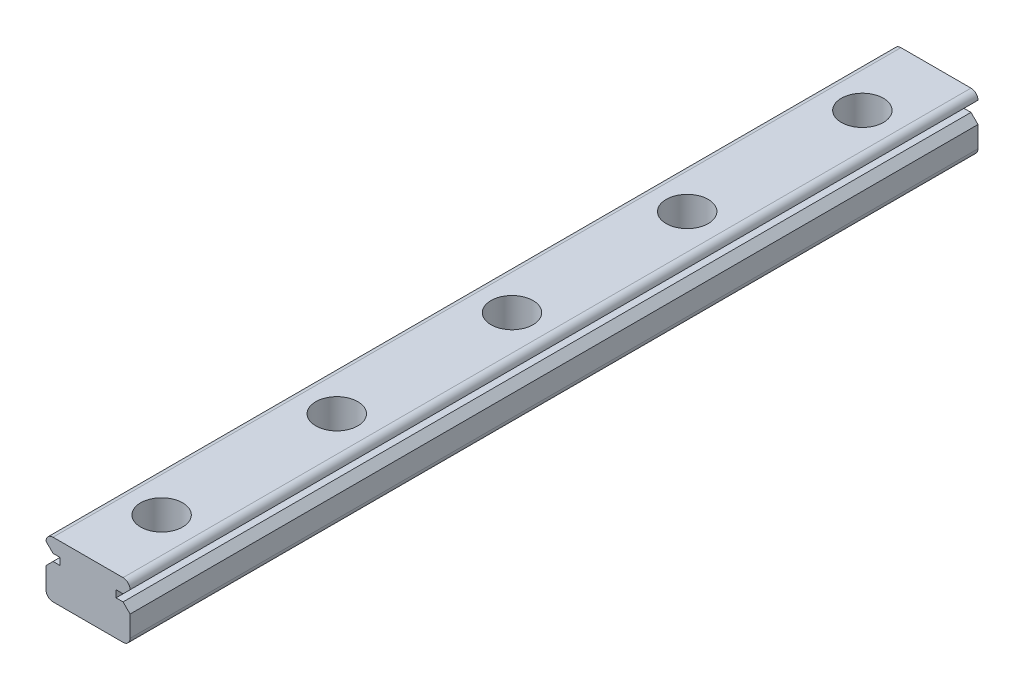
SolidWorks part; units mm, degrees
ref_plane "Front Plane" through (0, 0, 0) normal (0, 0, 1) x (1, 0, 0)
ref_plane "Top Plane" through (0, 0, 0) normal (0, 1, 0) x (1, 0, 0)
ref_plane "Right Plane" through (0, 0, 0) normal (1, 0, 0) x (0, 0, -1)
sketch "Sketch1" plane through (0, 0, 0) normal (0, 0, 1) x (1, 0, 0)
  line L0 (-8.4152, 2) -> (9.9405, 2) construction
  line L1 (-5, 4) -> (5, 4)
  line L2 (-5, 2) -> (-4, 2)
  line L3 (-5, -4) -> (5, -4)
  line L4 (6, 0) -> (6, -3)
  line L5 (-6, 4) -> (6, -4) construction
  line L6 (-6, -4) -> (6, 4) construction
  line L7 (-8.4152, 1) -> (9.9405, 1) construction
  line L8 (-4, 5.3337) -> (-4, -5.1622) construction
  line L9 (0, 4.6383) -> (0, -5.3401) construction
  line L10 (-5, 2) -> (-6, 3)
  line L11 (-5, 1) -> (-6, 0)
  line L12 (-6, 0) -> (-6, -3)
  line L13 (-4, 2) -> (-4, 1)
  line L14 (-4, 1) -> (-5, 1)
  line L15 (4, 1) -> (5, 1)
  line L16 (4, 2) -> (4, 1)
  line L17 (5, 1) -> (6, 0)
  line L18 (5, 2) -> (6, 3)
  line L19 (5, 2) -> (4, 2)
  arc A0 (-6, -3) -> (-5, -4) centre (-5, -3) ccw
  arc A1 (5, -4) -> (6, -3) centre (5, -3) ccw
  arc A2 (5, 4) -> (6, 3) centre (5, 3) cw
  arc A3 (-5, 4) -> (-6, 3) centre (-5, 3) ccw
  point P0 (0, 0)
  dimension "D3" = 1
  dimension "D1" = 12
  dimension "D2" = 8
  dimension "D4" = 1
  dimension "D5" = 2
extrude "Boss-Extrude1" add sketch "Sketch1" along normal blind 121
sketch "Sketch2" plane through (0, 4, 0) normal (0, 1, 0) x (1, 0, 0)
  line L0 (0, 0) -> (0, -121) construction
  line L1 (5, -121) -> (-5, -121) construction
  circle A0 centre (0, -10.5) radius 3
  circle A1 centre (0, -35.5) radius 3
  circle A2 centre (0, -60.5) radius 3
  circle A3 centre (0, -85.5) radius 3
  circle A4 centre (0, -110.5) radius 3
  dimension "D1" = 6
  dimension "D2" = 6
  dimension "D3" = 6
  dimension "D4" = 6
  dimension "D5" = 6
  dimension "D6" = 10.5
  dimension "D7" = 25
  dimension "D8" = 25
  dimension "D9" = 25
  dimension "D10" = 25
extrude "Cut-Extrude1" cut sketch "Sketch2" against normal blind 4.5
sketch "Sketch3" plane through (0, -0.5, 0) normal (0, 1, 0) x (1, 0, 0)
  circle A0 centre (0, -35.5) radius 1.75
  circle A1 centre (0, -10.5) radius 1.75
  circle A2 centre (0, -60.5) radius 1.75
  circle A3 centre (0, -85.5) radius 1.75
  circle A4 centre (0, -110.5) radius 1.75
  dimension "D1" = 3.5
  dimension "D2" = 3.5
  dimension "D3" = 3.5
  dimension "D4" = 3.5
  dimension "D5" = 3.5
extrude "Cut-Extrude2" cut sketch "Sketch3" against normal through all
